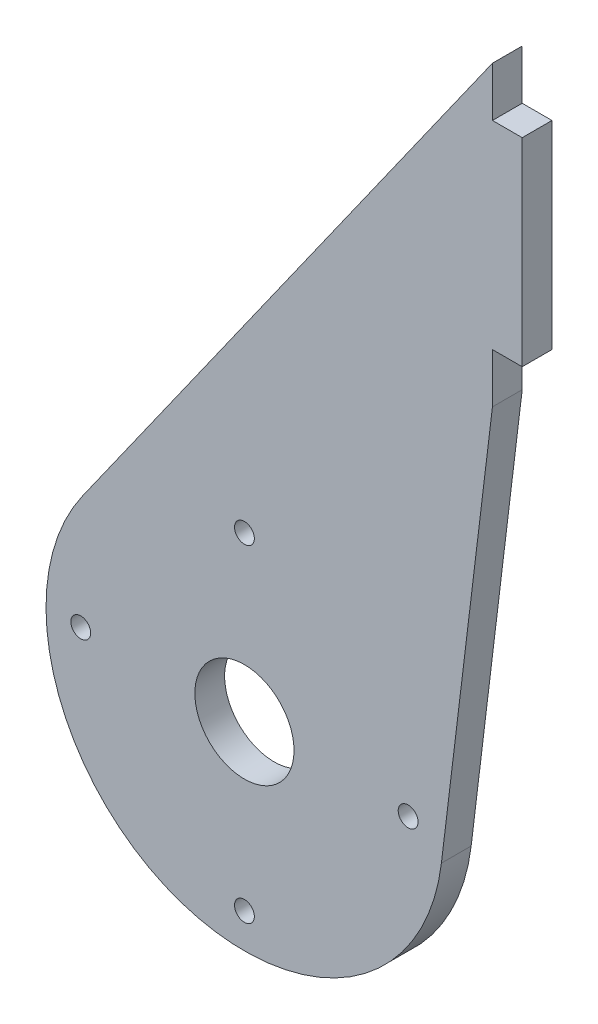
SolidWorks part; units mm, degrees
ref_plane "Front Plane" through (0, 0, 0) normal (0, 0, 1) x (1, 0, 0)
ref_plane "Top Plane" through (0, 0, 0) normal (0, 1, 0) x (1, 0, 0)
ref_plane "Right Plane" through (0, 0, 0) normal (1, 0, 0) x (0, 0, -1)
sketch "Sketch1" plane through (0, 0, 0) normal (0, 0, 1) x (1, 0, 0)
  line L0 (-16.3303, 11.5465) -> (25, 70)
  line L1 (25, 70) -> (25, 40)
  line L2 (25, 40) -> (19.8544, -2.409)
  line L3 (0, 0) -> (0, 52.3631) construction
  arc A0 (-16.3303, 11.5465) -> (19.8544, -2.409) centre (0, 0) ccw
  dimension "D6" = 20
  dimension "D7" = 25
  dimension "D8" = 70
  dimension "D9" = 30
  dimension "D10" = 6.918
extrude "Boss-Extrude1" add sketch "Sketch1" against normal blind 3
sketch "Sketch2" plane through (0, 0, 0) normal (0, 0, 1) x (1, 0, 0)
  circle A0 centre (0, 0) radius 5
  dimension "D1" = 10
extrude "Cut-Extrude1" cut sketch "Sketch2" against normal blind 10
sketch "Sketch4" plane through (25, 0, 0) normal (1, 0, 0) x (0, 0, -1)
  line L0 (0, 40) -> (0, 70) construction
  line L1 (0, 65) -> (3, 65)
  line L2 (0, 65) -> (0, 45)
  line L3 (0, 45) -> (3, 45)
  line L4 (3, 65) -> (3, 45)
  line L5 (3, 40) -> (3, 70) construction
  line L6 (3, 40) -> (0, 40) construction
  dimension "D1" = 20
  dimension "D2" = 5
extrude "Boss-Extrude3" add sketch "Sketch4" along normal blind 3
sketch "Sketch5" plane through (0, 0, 0) normal (0, 0, 1) x (1, 0, 0)
  circle A0 centre (0, 16.5) radius 1
  circle A1 centre (0, -16.5) radius 1
  circle A2 centre (16.5, 0) radius 1
  circle A3 centre (-16.5, 0) radius 1
  circle A4 centre (0, 0) radius 5 construction
  dimension "D1" = 16.5
  dimension "D2" = 2
  dimension "D3" = 16.5
  dimension "D4" = 2
  dimension "D5" = 16.5
  dimension "D6" = 2
  dimension "D7" = 16.5
  dimension "D8" = 2
extrude "Cut-Extrude2" cut sketch "Sketch5" against normal blind 10
